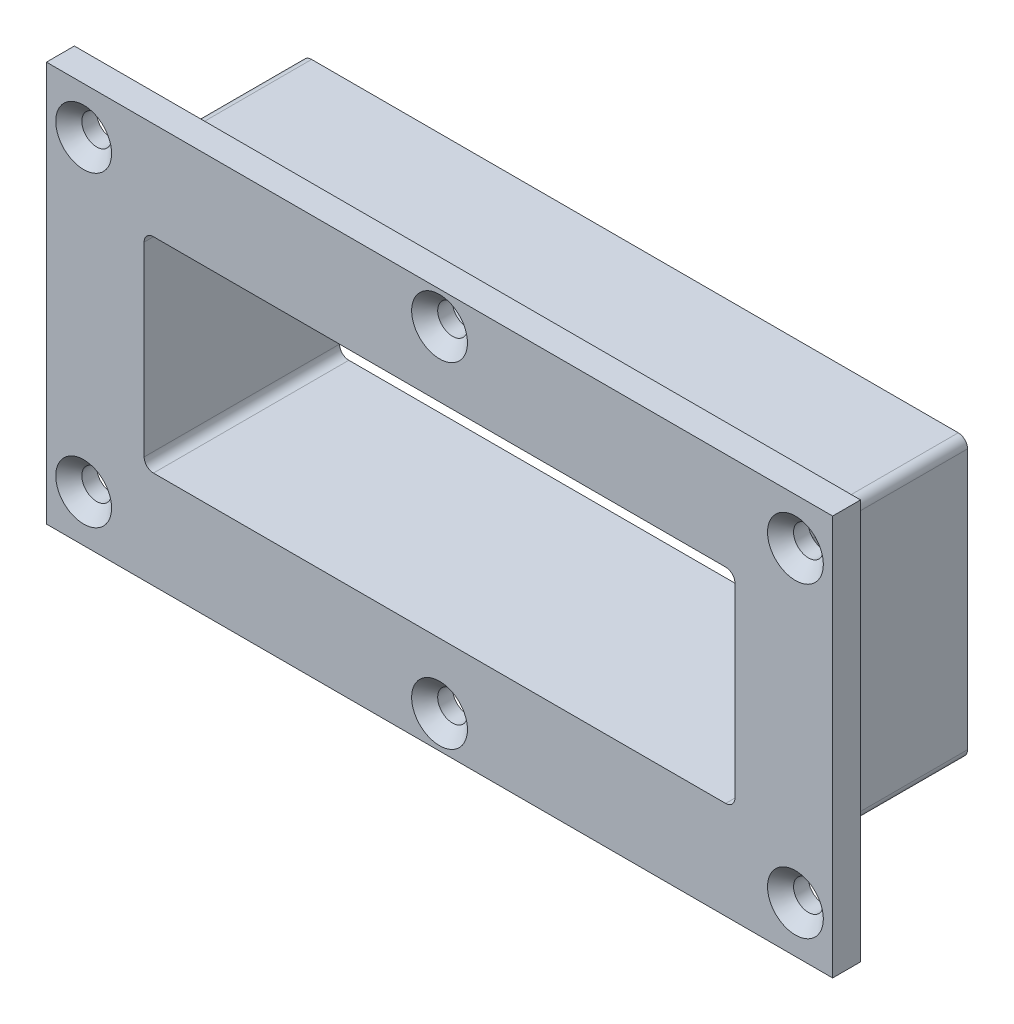
SolidWorks part; units mm, degrees
ref_plane "Front Plane" through (0, 0, 0) normal (0, 0, 1) x (1, 0, 0)
ref_plane "Top Plane" through (0, 0, 0) normal (0, 1, 0) x (1, 0, 0)
ref_plane "Right Plane" through (0, 0, 0) normal (1, 0, 0) x (0, 0, -1)
sketch "Sketch1" plane through (0, 0, 0) normal (0, 0, 1) x (1, 0, 0)
  line L0 (-35.75, -15) -> (-35.75, 15)
  line L1 (31.75, -11) -> (-31.75, -11)
  line L2 (31.75, -11) -> (31.75, 11)
  line L3 (31.75, 11) -> (-31.75, 11)
  line L4 (-31.75, -11) -> (-31.75, 11)
  line L5 (31.75, -11) -> (-31.75, 11) construction
  line L6 (31.75, 11) -> (-31.75, -11) construction
  line L7 (35.75, 15) -> (-35.75, 15)
  line L8 (35.75, -15) -> (35.75, 15)
  line L9 (35.75, -15) -> (-35.75, -15)
  point P0 (0, 0)
  dimension "D1" = 22
  dimension "D2" = 63.5
  dimension "D3" = 4
extrude "Boss-Extrude1" add sketch "Sketch1" along normal blind 21
sketch "Sketch2" plane through (0, 0, 21) normal (0, 0, 1) x (1, 0, 0)
  line L0 (35.75, 15) -> (42.25, 15) construction
  line L1 (42.25, 15) -> (42.25, -15)
  line L2 (42.25, -15) -> (35.75, -15) construction
  line L3 (-35.75, 15) -> (-42.25, 15) construction
  line L4 (-35.75, -15) -> (35.75, -15)
  line L5 (35.75, -15) -> (35.75, 15)
  line L6 (35.75, 15) -> (-35.75, 15)
  line L7 (-35.75, 15) -> (-35.75, -15)
  line L9 (35.75, -15) -> (35.75, 15) construction
  line L11 (-35.75, 15) -> (-35.75, -15) construction
  line L12 (-42.25, 15) -> (-42.25, -15)
  line L13 (-42.25, -15) -> (-35.75, -15) construction
  line L14 (-42.25, 15) -> (-42.25, 21.5)
  line L15 (-42.25, 21.5) -> (42.25, 21.5)
  line L16 (42.25, 21.5) -> (42.25, 15)
  line L17 (42.25, -15) -> (42.25, -21.5)
  line L18 (42.25, -21.5) -> (-42.25, -21.5)
  line L19 (-42.25, -21.5) -> (-42.25, -15)
  line L24 (-35.75, -15) -> (35.75, -15)
  line L25 (-35.75, 15) -> (-35.75, -15)
  line L26 (35.75, 15) -> (-35.75, 15)
  line L27 (35.75, -15) -> (35.75, 15)
  line L28 (-35.75, -15) -> (35.75, -15)
  line L29 (-35.75, 15) -> (-35.75, -15)
  line L30 (35.75, 15) -> (-35.75, 15)
  line L31 (35.75, -15) -> (35.75, 15)
  dimension "D2" = 6.5
  dimension "D3" = 6.5
  dimension "D4" = 6.5
  dimension "D5" = 6.5
  dimension "D6" = 0
  dimension "D1" = 0
extrude "Boss-Extrude2" add sketch "Sketch2" against normal blind 3
sketch "Sketch3" plane through (0, 0, 0) normal (0, 0, -1) x (-1, 0, 0)
  line L10 (-34.45, 13.7) -> (-34.45, -13.7)
  line L11 (-34.45, -13.7) -> (34.45, -13.7)
  line L12 (34.45, -13.7) -> (34.45, 13.7)
  line L13 (34.45, 13.7) -> (-34.45, 13.7)
  line L14 (32.95, -12.2) -> (32.95, 12.2)
  line L15 (-32.95, -12.2) -> (32.95, -12.2)
  line L16 (32.95, 12.2) -> (-32.95, 12.2)
  line L17 (-32.95, 12.2) -> (-32.95, -12.2)
  line L18 (32.95, -12.2) -> (32.95, 12.2)
  line L19 (-32.95, -12.2) -> (32.95, -12.2)
  line L20 (32.95, 12.2) -> (-32.95, 12.2)
  line L21 (-32.95, 12.2) -> (-32.95, -12.2)
  dimension "D1" = 1.2
  dimension "D2" = 1.5
extrude "Cut-Extrude1" cut sketch "Sketch3" against normal blind 1.5
sketch "Sketch4" plane through (0, 0, 18) normal (0, 0, -1) x (-1, 0, 0)
  line L0 (0, 0) -> (0, 29.1662) construction
  line L1 (-42.25, -21.5) -> (-42.25, 21.5) construction
  line L5 (42.25, -21.5) -> (-42.25, -21.5) construction
  line L6 (-42.25, 21.5) -> (42.25, 21.5) construction
  circle A0 centre (-38.25, 16.5) radius 1.6
  circle A1 centre (-38.25, -16.5) radius 1.6
  circle A2 centre (38.25, -16.5) radius 1.6
  circle A3 centre (38.25, 16.5) radius 1.6
  circle A4 centre (0, -18) radius 1.6
  circle A5 centre (0, 18) radius 1.6
  dimension "D1" = 3.2
  dimension "D2" = 3.2
  dimension "D6" = 3.2
  dimension "D7" = 3.2
  dimension "D3" = 4
  dimension "D4" = 5
  dimension "D5" = 5
extrude "Cut-Extrude2" cut sketch "Sketch4" against normal blind 3
hole_wizard "Pilot hole size (% per cross) for half-countersunk wood screw, type 1" positions "Sketch5" profile "Sketch6" countersink size "M3" standard "GB"
sketch "Sketch5" plane through (0, 0, 21) normal (0, 0, 1) x (1, 0, 0)
  point P0 (-38.25, 16.5)
  point P3 (-38.25, -16.5)
  point P6 (38.25, 16.5)
  point P9 (38.25, -16.5)
  point P12 (0, -18)
  point P15 (0, 18)
sketch "Sketch6" plane through (-38.25, 16.5, 21) normal (1, 0, 0) x (0, -1, 0)
  line L0 (0, 0) -> (0, 7.0614)
  line L1 (0, 7.0614) -> (1.6, 6.1)
  line L2 (1.6, 6.1) -> (1.6, 1.4)
  line L3 (1.6, 1.4) -> (3, 0)
  line L5 (3, 0) -> (0, 0)
  line L6 (-1.6, 1.4) -> (-3, 0) construction
  line L10 (0, 7.0614) -> (-1.6, 6.1) construction
  line L11 (0, -6.35) -> (0, 107.95) construction
  dimension "孔直径" = 3.2
  dimension "孔深度" = 6.1
  dimension "近端锥形沉头孔直径" = 6
  dimension "近端锥形沉头孔角度" = 90
  dimension "导头角度" = 118
fillet "Fillet1" radius 1 12 edges at (31.75, 11, 10.5) (-31.75, 11, 10.5) (-31.75, -11, 10.5) (31.75, -11, 10.5) (32.95, -12.2, 0.75) (32.95, 12.2, 0.75) (-32.95, 12.2, 0.75) (-32.95, -12.2, 0.75) (34.45, -13.7, 0.75) (34.45, 13.7, 0.75) (-34.45, 13.7, 0.75) (-34.45, -13.7, 0.75)
fillet "Fillet2" radius 1 4 edges at (35.75, -15, 9) (35.75, 15, 9) (-35.75, 15, 9) (-35.75, -15, 9)
